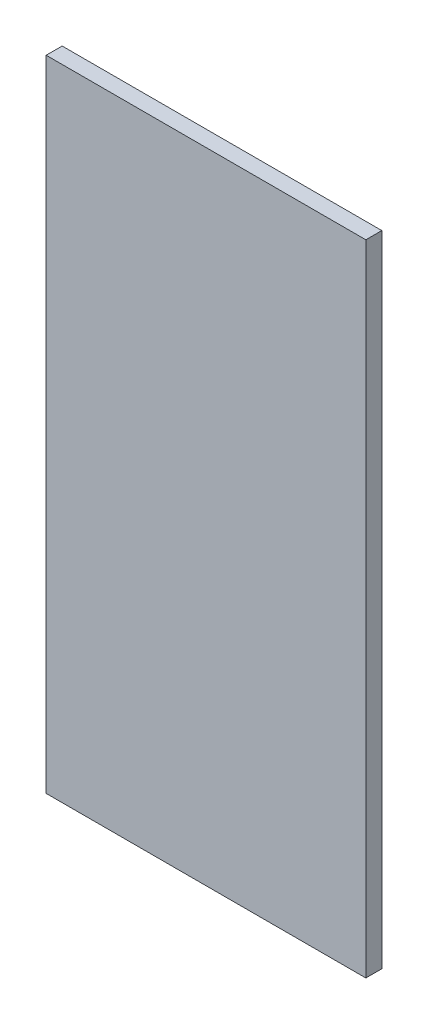
SolidWorks part; units mm, degrees
ref_plane "Front Plane" through (0, 0, 0) normal (0, 0, 1) x (1, 0, 0)
ref_plane "Top Plane" through (0, 0, 0) normal (0, 1, 0) x (1, 0, 0)
ref_plane "Right Plane" through (0, 0, 0) normal (1, 0, 0) x (0, 0, -1)
other "Configuration Table"
sketch "Sketch1" plane through (0, 0, 0) normal (0, 0, 1) x (1, 0, 0)
  line L1 (-300, -600) -> (300, -600)
  line L2 (-300, -600) -> (-300, 600)
  line L3 (-300, 600) -> (300, 600)
  line L4 (300, -600) -> (300, 600)
  line L5 (-300, -600) -> (300, 600) construction
  line L6 (-300, 600) -> (300, -600) construction
  point P0 (0, 0)
  dimension "D1" = 600
  dimension "D2" = 1200
extrude "Boss-Extrude1" add sketch "Sketch1" along normal blind 30
sketch "Sketch2" plane through (0, 0, 0) normal (0, 0, -1) x (-1, 0, 0)
  line L0 (0, 600) -> (0, -600) construction
  line L1 (-300, 600) -> (300, 600) construction
  line L2 (300, -600) -> (-300, -600) construction
  line L3 (-300, 0) -> (300, 0) construction
  line L4 (-300, -600) -> (-300, 600) construction
  line L5 (300, 600) -> (300, -600) construction
  circle A0 centre (-180, 480) radius 60
  circle A1 centre (180, 480) radius 60
  circle A2 centre (180, -480) radius 60
  circle A3 centre (-180, -480) radius 60
  dimension "D1" = 120
  dimension "D2" = 180
  dimension "D3" = 120
extrude "Cut-Extrude1" cut sketch "Sketch2" against normal blind 2
